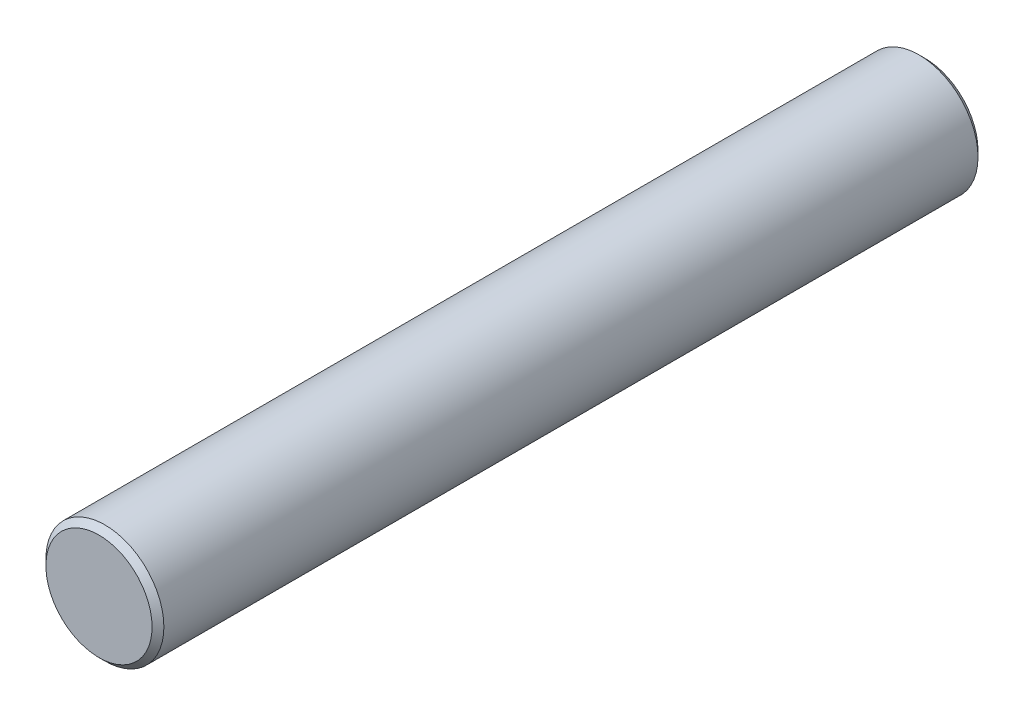
from build123d import *

# Parameters (mm, degrees)
SKETCH1_R           = 10
BOSS_EXTRUDE1_DEPTH = 140
CHAMFER2_SIZE       = 1


with BuildPart() as part:
    # Sketch1 → Boss-Extrude1 (new body)
    with BuildSketch(Plane.XY):
        Circle(SKETCH1_R)
    extrude(amount=-BOSS_EXTRUDE1_DEPTH)

    # Chamfer2
    chamfer2_edges = [part.edges().sort_by_distance(p)[0] for p in [
        (-10, 0, 0),
        (-10, 0, -140),
    ]]
    chamfer(chamfer2_edges, length=CHAMFER2_SIZE)


solid = part.part
